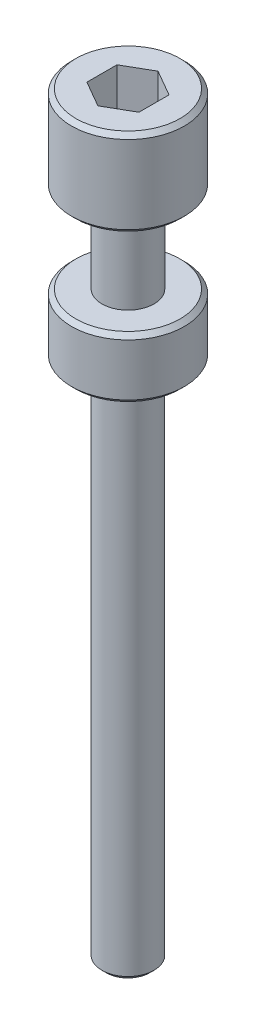
SolidWorks part; units mm, degrees
ref_plane "Front Plane" through (0, 0, 0) normal (0, 0, 1) x (1, 0, 0)
ref_plane "Top Plane" through (0, 0, 0) normal (0, 1, 0) x (1, 0, 0)
ref_plane "Right Plane" through (0, 0, 0) normal (1, 0, 0) x (0, 0, -1)
sketch "Sketch1" plane through (0, 0, 0) normal (0, 1, 0) x (1, 0, 0)
  circle A0 centre (0, 0) radius 3
  dimension "D1" = 6
extrude "Boss-Extrude1" add sketch "Sketch1" along normal blind 45
cosmetic thread "Cosmetic Thread1" parameters "D1"=50, "D2"=5.5
sketch "Sketch2" plane through (0, 45, 0) normal (0, 1, 0) x (1, 0, 0)
  circle A0 centre (0, 0) radius 3
  dimension "D1" = 6
extrude "Boss-Extrude2" add sketch "Sketch2" along normal blind 15
sketch "Sketch3" plane through (0, 60, 0) normal (0, 1, 0) x (1, 0, 0)
  circle A0 centre (0, 0) radius 6.5
  dimension "D1" = 13
extrude "Boss-Extrude3" add sketch "Sketch3" along normal blind 7
sketch "Sketch4" plane through (0, 67, 0) normal (0, 1, 0) x (1, 0, 0)
  circle A0 centre (0, 0) radius 3 construction
  circle A1 centre (0, 0) radius 3
extrude "Boss-Extrude4" add sketch "Sketch4" along normal blind 10
sketch "Sketch5" plane through (0, 77, 0) normal (0, 1, 0) x (1, 0, 0)
  circle A0 centre (0, 0) radius 6.5
  dimension "D1" = 13
extrude "Boss-Extrude5" add sketch "Sketch5" along normal blind 10
sketch "Sketch6" plane through (0, 87, 0) normal (0, 1, 0) x (1, 0, 0)
  line L1 (0, 3.4641) -> (-3, 1.7321)
  line L2 (-3, 1.7321) -> (-3, -1.7321)
  line L3 (-3, -1.7321) -> (0, -3.4641)
  line L4 (0, -3.4641) -> (3, -1.7321)
  line L5 (3, -1.7321) -> (3, 1.7321)
  line L6 (3, 1.7321) -> (0, 3.4641)
  circle A0 centre (0, 0) radius 3 construction
  dimension "D1" = 6
extrude "Cut-Extrude1" cut sketch "Sketch6" against normal blind 6
chamfer "Chamfer1" distance 0.5 angle 45 5 edges at (0, 60, 6.5) (0, 67, 6.5) (0, 87, 6.5) (0, 77, 6.5) (0, 0, 3)
